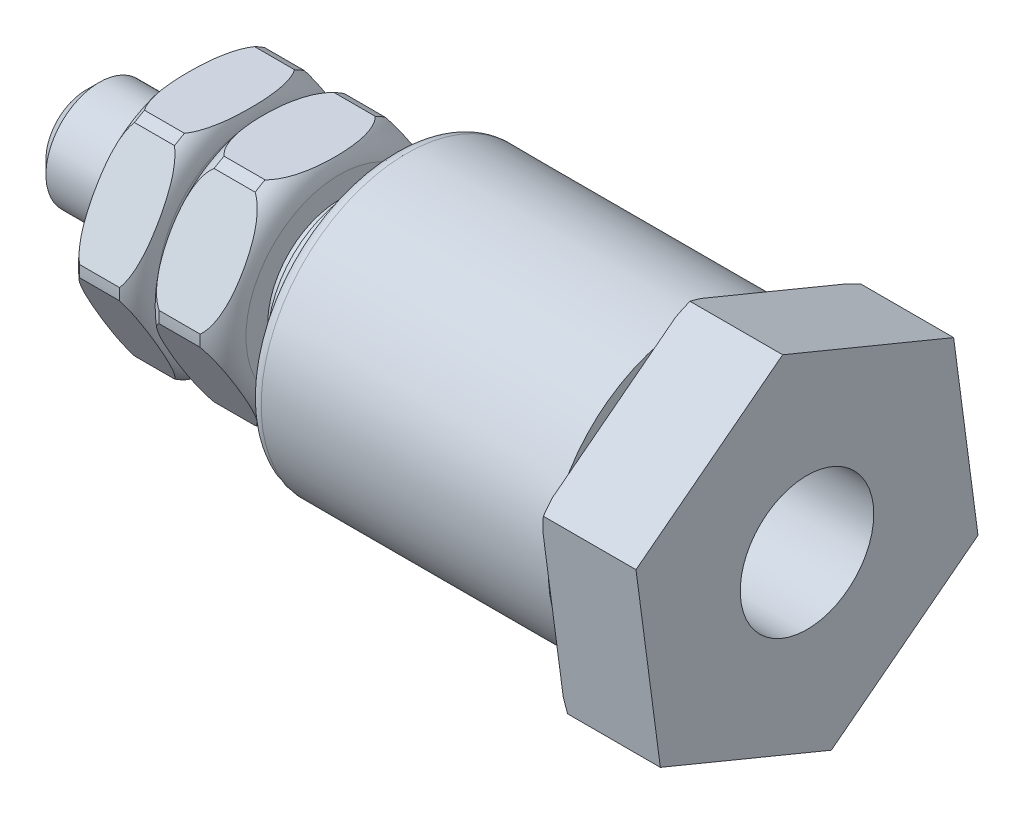
SolidWorks part; units mm, degrees
ref_plane "Front Plane" through (0, 0, 0) normal (0, 0, 1) x (1, 0, 0)
ref_plane "Top Plane" through (0, 0, 0) normal (0, 1, 0) x (1, 0, 0)
ref_plane "Right Plane" through (0, 0, 0) normal (1, 0, 0) x (0, 0, -1)
sketch "Sketch1" plane through (0, 0, 0) normal (0, 0, 1) x (1, 0, 0)
  line L0 (10.5531, 13.3323) -> (10.5531, 9.121)
  line L1 (-27.8179, 9) -> (-24.8179, 9)
  line L2 (-23.8179, 7.125) -> (-23.8179, 5.5)
  line L3 (-23.8179, 5.5) -> (-23.3179, 5.5)
  line L4 (-23.3179, 5.5) -> (-23.3179, 6.0187)
  line L5 (-21.8546, 9) -> (-18.7813, 9)
  line L6 (-17.3179, 7.0187) -> (-17.3179, 5.3937)
  line L7 (-17.3179, 5.3937) -> (-16.3179, 5.3937)
  line L8 (-16.3179, 5.3937) -> (-16.3179, 6.3937)
  line L9 (-16.3179, 6.3937) -> (-15.3179, 6.3937)
  line L10 (-15.3179, 6.3937) -> (-15.3179, 5.3937)
  line L11 (-15.3179, 5.3937) -> (-13.3179, 9.3937)
  line L12 (-13.3179, 9.3937) -> (-13.3179, 9.8937)
  line L13 (-12.3045, 10.8936) -> (9.1955, 10.8937)
  line L14 (9.1955, 10.8937) -> (9.1955, 9.121)
  line L15 (10.5531, 9.121) -> (9.1955, 9.121)
  line L16 (17.6821, 5) -> (17.6821, 14.0459)
  line L19 (17.6821, 5) -> (-4.3406, 5)
  line L20 (-4.3406, 5) -> (-7, 0)
  line L21 (-7, 0) -> (-36.3179, 0)
  line L22 (-36.3179, 0) -> (-36.3179, 3)
  line L23 (-36.3179, 3) -> (-35.3179, 4)
  line L24 (-35.3179, 4) -> (-28.8179, 4)
  line L25 (-28.8179, 4) -> (-28.8179, 7.125)
  arc A0 (-23.8179, 7.125) -> (-24.8179, 9) centre (-26.0757, 7.125) ccw
  arc A1 (-21.8546, 9) -> (-23.3179, 6.0187) centre (-20.9225, 6.6927) ccw
  arc A2 (-17.3179, 7.0187) -> (-18.7813, 9) centre (-19.789, 6.7247) ccw
  arc A3 (-12.3045, 10.8936) -> (-13.3179, 9.8937) centre (-12.3179, 9.8937) ccw
  arc A5 (17.6821, 14.0459) -> (10.5531, 13.3323) centre (14.2589, 12.2766) ccw
  arc A6 (-27.8179, 9) -> (-28.8179, 7.125) centre (-26.5601, 7.125) ccw
  dimension "D1" = 9
  dimension "D2" = 9
  dimension "D3" = 5
  dimension "D4" = 54
  dimension "D5" = 19
  dimension "D6" = 21.5
  dimension "D7" = 0
revolve "Revolve1" add sketch "Sketch1" angle 360 about L21
sketch "Sketch2" plane through (-28.8179, 0, 0) normal (-1, 0, 0) x (0, 0, 1)
  line L0 (-4.6188, 8) -> (4.6188, 8)
  line L1 (-11.7886, 0) -> (12.4629, 0) construction
  line L2 (4.6188, 8) -> (9.2376, 0)
  line L3 (9.2376, 0) -> (4.6188, -8)
  line L4 (4.6188, -8) -> (-4.6188, -8)
  line L5 (-4.6188, -8) -> (-9.2376, 0)
  line L6 (-9.2376, 0) -> (-4.6188, 8)
  circle A0 centre (0, 0) radius 13.3402
  dimension "D1" = 8
extrude "Cut-Extrude1" cut sketch "Sketch2" against normal up to surface (11.5 mm away) up to face at (-17.3179, 0, -7.0187)
sketch "Sketch4" plane through (17.6821, 0, 0) normal (1, 0, 0) x (0, 0, -1)
  line L1 (12.8074, -5.2888) -> (10.9839, 8.4471)
  line L2 (10.9839, 8.4471) -> (-1.8235, 13.7359)
  line L3 (-1.8235, 13.7359) -> (-12.8074, 5.2888)
  line L4 (-12.8074, 5.2888) -> (-10.9839, -8.4471)
  line L5 (-10.9839, -8.4471) -> (1.8235, -13.7359)
  line L6 (1.8235, -13.7359) -> (12.8074, -5.2888)
  circle A0 centre (0, 0) radius 12 construction
  dimension "D1" = 24
extrude "Cut-Extrude3" cut sketch "Sketch4" against normal blind 20 flip side to cut
